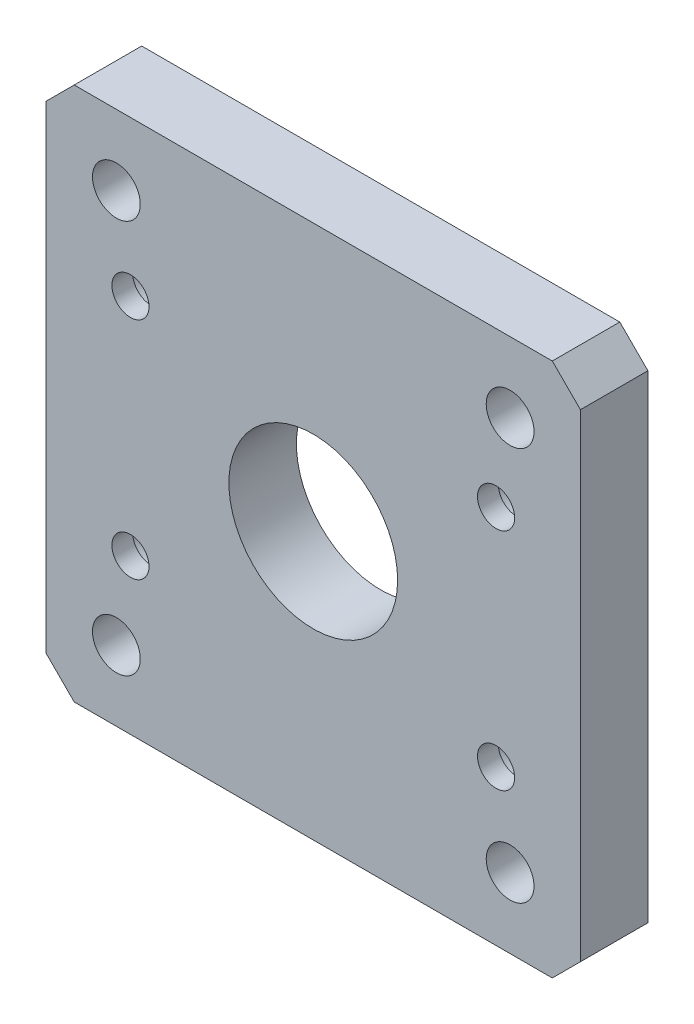
from build123d import *

# Parameters (mm, degrees)
SKETCH_1_W                = 95
SKETCH_1_H                = 95
EXTRUDE_1_DEPTH           = 12
SKETCH_2_R                = 15
CUT_EXTRUDE_1_DEPTH       = 108.604604424
HOLE_WIZARD_1_D           = 6.6
HOLE_WIZARD_1_CBORE_D     = 11
HOLE_WIZARD_1_CBORE_DEPTH = 8.3
HOLE_WIZARD_M10_2_D       = 8.5
CHAMFER_1_SIZE            = 5


with BuildPart() as part:
    # 草图1 → 凸台-拉伸1 (new body)
    with BuildSketch(Plane.XY):
        with Locations((48.304493075, 0)):
            Rectangle(SKETCH_1_W, SKETCH_1_H)
    extrude(amount=EXTRUDE_1_DEPTH)

    # 草图2 → 切除-拉伸1 (cut, through all)
    with BuildSketch(Plane.XY.offset(12)):
        with Locations((48.304493075, 0)):
            Circle(SKETCH_2_R)
    extrude(amount=-CUT_EXTRUDE_1_DEPTH, mode=Mode.SUBTRACT)

    # 打孔尺寸(%根据)内六角圆柱头螺钉的类型1 (through all)
    with Locations(Plane(origin=(80.804493075, 20, 0), x_dir=(-1, 0, 0), z_dir=(0, 0, -1))):
        with Locations((0, 0), (65, 0), (65, -40), (0, -40)):
            CounterBoreHole(HOLE_WIZARD_1_D / 2, HOLE_WIZARD_1_CBORE_D / 2, HOLE_WIZARD_1_CBORE_DEPTH)

    # M10 螺纹孔2 (through all)
    with Locations(Plane(origin=(83.304493075, 35, 0), x_dir=(-1, 0, 0), z_dir=(0, 0, -1))):
        with Locations((0, 0), (70, 0), (70, -70), (0, -70)):
            Hole(HOLE_WIZARD_M10_2_D / 2)

    # 倒角1
    chamfer_1_edges = [part.edges().sort_by_distance(p)[0] for p in [
        (0.804493075, 47.5, 6),
        (95.804493075, 47.5, 6),
        (95.804493075, -47.5, 6),
        (0.804493075, -47.5, 6),
    ]]
    chamfer(chamfer_1_edges, length=CHAMFER_1_SIZE)


solid = part.part
